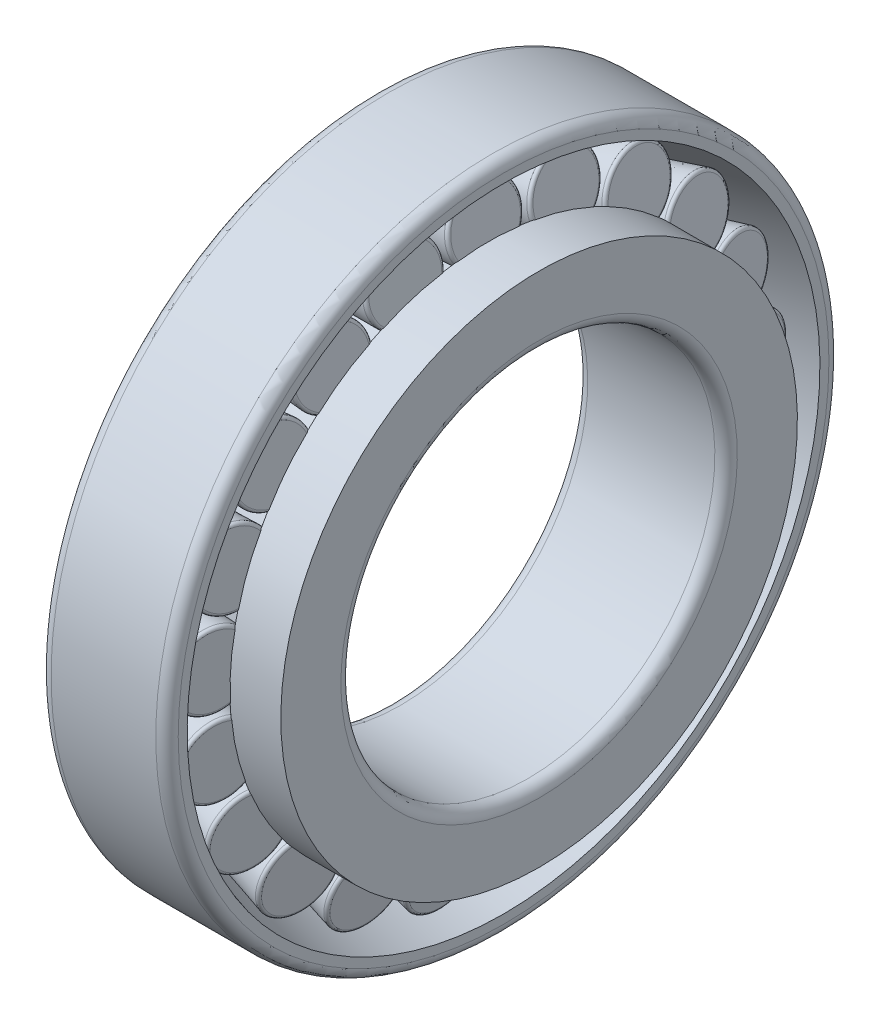
SolidWorks part; units mm, degrees
ref_plane "Front" through (0, 0, 0) normal (0, 0, 1) x (1, 0, 0)
ref_plane "Top" through (0, 0, 0) normal (0, 1, 0) x (1, 0, 0)
ref_plane "Right" through (0, 0, 0) normal (1, 0, 0) x (0, 0, -1)
sketch "Sketch1" plane through (0, 0, 0) normal (0, 0, 1) x (1, 0, 0)
  line L0 (13.25, 0) -> (13.9916, 0) construction
  line L1 (8.5, 42.2989) -> (8.5, 43.5)
  line L2 (7, 45) -> (-7, 45)
  line L3 (-8.5, 43.5) -> (-8.5, 37.539)
  line L4 (-8.5, 37.539) -> (8.5, 42.2989)
  line L5 (-6.75, 26.5) -> (-6.75, 31.9296)
  line L6 (-5.25, 25) -> (11.75, 25)
  line L7 (13.25, 26.5) -> (13.25, 34.5339)
  line L8 (-4.1773, 30.4296) -> (-5.6625, 38.3335)
  line L9 (7, 31.5339) -> (5.1533, 41.3619)
  line L10 (-4.9199, 34.3816) -> (6.0766, 36.4479) construction
  line L11 (-4.1773, 30.4296) -> (7, 31.5339)
  line L12 (6.4363, 35) -> (13.25, 35)
  line L13 (13.25, 34.5339) -> (6.4363, 34.5339)
  line L14 (-6.75, 31.9296) -> (-4.4592, 31.9296)
  arc A0 (-7, 45) -> (-8.5, 43.5) centre (-7, 43.5) ccw
  arc A1 (8.5, 43.5) -> (7, 45) centre (7, 43.5) ccw
  arc A2 (-5.25, 25) -> (-6.75, 26.5) centre (-5.25, 26.5) cw
  arc A3 (11.75, 25) -> (13.25, 26.5) centre (11.75, 26.5) ccw
  point P19 (-8.5, 45)
  point P22 (8.5, 45)
  point P24 (0, 45)
  point P29 (-6.75, 25)
  point P32 (13.25, 25)
revolve "Revolve1" add sketch "Sketch1" angle 360 about L0
sketch "Sketch2" plane through (0, 0, 0) normal (0, 0, 1) x (1, 0, 0)
  line L0 (-4.9396, 34.3779) -> (7.5076, 36.7167) construction
  line L4 (-4.9199, 34.3816) -> (6.0766, 36.4479) construction
  line L5 (-4.9396, 34.3779) -> (6.0963, 36.4515)
  line L7 (-5.6822, 38.3298) -> (-4.1936, 30.4079)
  line L8 (7.0237, 31.5161) -> (5.1729, 41.3655)
  line L9 (-4.1936, 30.4079) -> (7.0237, 31.5161)
  line L10 (-4.9396, 34.3779) -> (-4.2613, 30.7682)
  line L11 (6.9431, 31.9451) -> (6.0963, 36.4515)
  line L12 (-3.8289, 30.444) -> (6.5893, 31.4732)
  arc A0 (-3.8289, 30.444) -> (-4.2613, 30.7682) centre (-3.8682, 30.842) cw
  arc A1 (6.5893, 31.4732) -> (6.9431, 31.9451) centre (6.55, 31.8712) ccw
revolve "Revolve2" add sketch "Sketch2" angle 360 about L0
sketch "Sketch3" plane through (0, 0, 0) normal (0, 0, 1) x (1, 0, 0)
  line L0 (-8.5, 37.539) -> (8.5, 42.2989) construction
  line L1 (-8.5, 43.5) -> (-8.5, 37.539) construction
  line L2 (7, 45) -> (-7, 45) construction
  line L3 (8.5, 42.2989) -> (8.5, 43.5) construction
  line L4 (-8.5, 37.539) -> (8.5, 42.2989)
  line L5 (-8.5, 43.5) -> (-8.5, 37.539)
  line L6 (7, 45) -> (-7, 45)
  line L7 (8.5, 42.2989) -> (8.5, 43.5)
  arc A0 (-7, 45) -> (-8.5, 43.5) centre (-7, 43.5) ccw construction
  arc A1 (8.5, 43.5) -> (7, 45) centre (7, 43.5) ccw construction
  arc A2 (-7, 45) -> (-8.5, 43.5) centre (-7, 43.5) ccw
  arc A3 (8.5, 43.5) -> (7, 45) centre (7, 43.5) ccw
revolve "Revolve3" add sketch "Sketch3" angle 360 about axis through (13.25, 0, 0) along (1, 0, 0)
pattern_circular "Circular-Pattern1" count 21 over 360 about axis through (0, 0, 0) along (1, 0, 0) of "Revolve2"
equation "\"gzzj@Sketch1\" =  ( \"DD@Sketch1\" - \"XD@Sketch1\" )  / 4"
equation "\"D1@Sketch1\" = \"DB@Sketch1\" - \"DT@Sketch1\" / 20"
equation "\"D2@Sketch1\" = \"DT@Sketch1\" - \"DC@Sketch1\" + \"XR12@Sketch1\""
equation "\"D4@Sketch1\" = \"D3@Sketch1\" / 2"
equation "\"D2@Sketch2\" = \"gzzj@Sketch1\" / 25"
equation "\"ZJ@Sketch1\" =  ( \"DD@Sketch1\" + \"XD@Sketch1\" )  / 2"
equation "\"D1@Circular-Pattern1\" = int( 3.14159265 / atn(( \"gzzj@Sketch1\" / 2) / sqr( \"ZJ@Sketch1\" * \"ZJ@Sketch1\" /4 - ( \"gzzj@Sketch1\"/ 2) *  ( \"gzzj@Sketch1\"/ 2))))"
